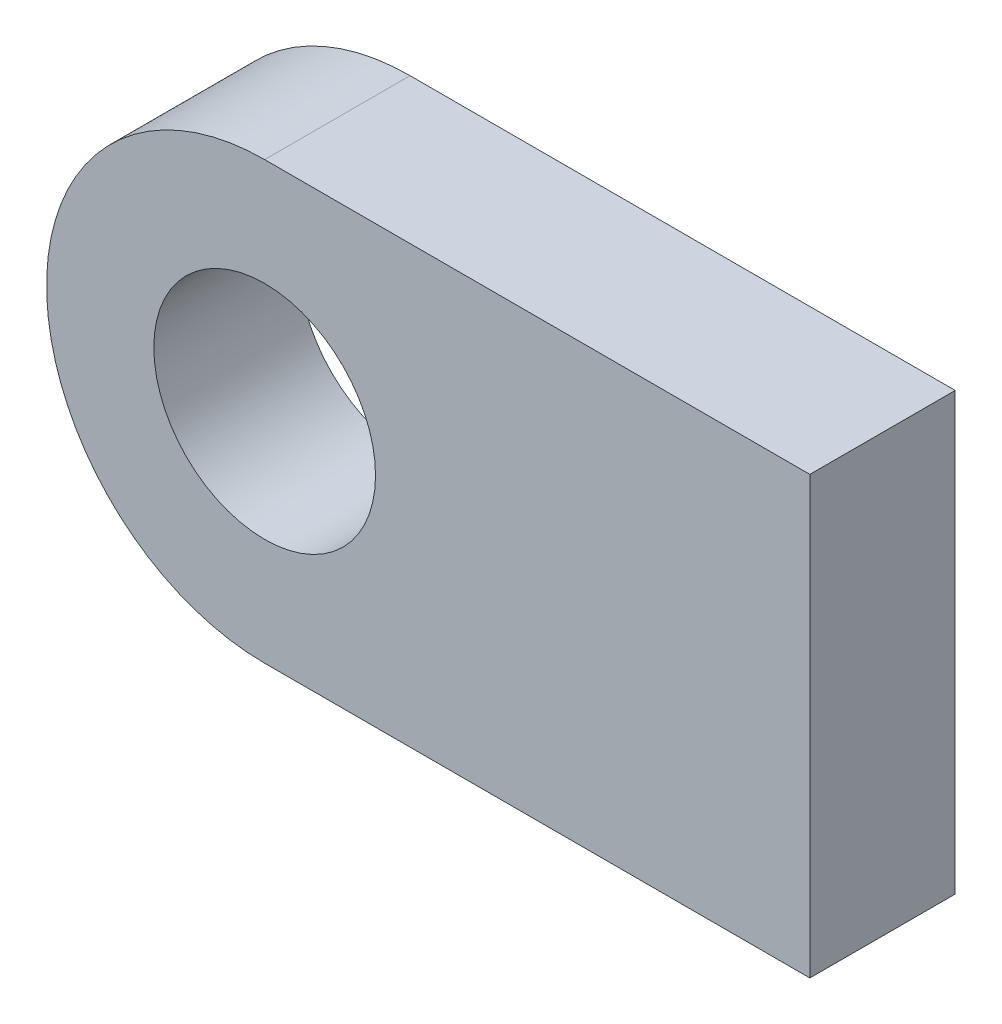
from build123d import *

# Parameters (mm, degrees)
SKETCH_1_R      = 6.1
EXTRUDE_1_DEPTH = 4


with BuildPart() as part:
    # 草图1 → 凸台-拉伸1 (new, symmetric)
    with BuildSketch(Plane.XY):
        with BuildLine():
            Line((0, 12), (30, 12))
            Line((30, 12), (30, -12))
            Line((30, -12), (0, -12))
            ThreePointArc((0, -12), (-12, 0), (0, 12))
        make_face()
        Circle(SKETCH_1_R, mode=Mode.SUBTRACT)
    extrude(amount=EXTRUDE_1_DEPTH, both=True)


solid = part.part
